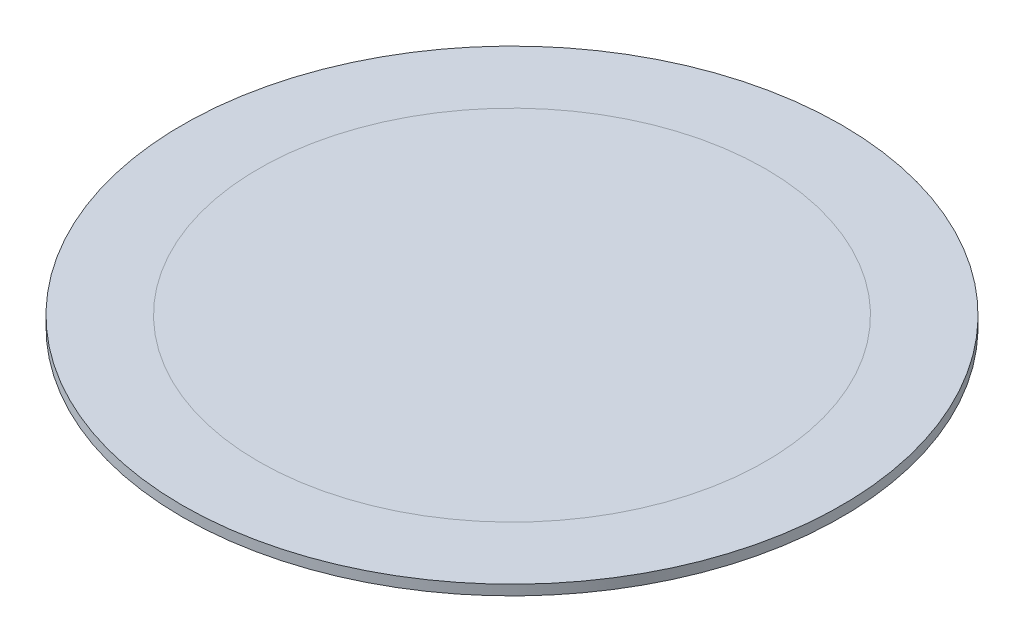
from build123d import *

# Parameters (mm, degrees)
SKETCH1_R           = 32.5
SKETCH1_R_2         = 25
BOSS_EXTRUDE1_DEPTH = 1
SKETCH2_R           = 25
BOSS_EXTRUDE2_DEPTH = 1


with BuildPart() as part:
    # Sketch1 → Boss-Extrude1 (new body)
    with BuildSketch(Plane(origin=(0, 0, 0), x_dir=(1, 0, 0), z_dir=(0, 1, 0))):
        with Locations(Location((0, 0, 0), (0, 0, 270))):
            Circle(SKETCH1_R)
        with Locations(Location((0, 0, 0), (0, 0, 270))):
            Circle(SKETCH1_R_2, mode=Mode.SUBTRACT)
    extrude(amount=BOSS_EXTRUDE1_DEPTH)


with BuildPart() as body_2:
    # Sketch2 → Boss-Extrude2 (new body)
    with BuildSketch(Plane.XZ):
        with Locations(Location((0, 0, 0), (0, 0, 270))):
            Circle(SKETCH2_R)
    extrude(amount=-BOSS_EXTRUDE2_DEPTH)


solid = Compound([part.part, body_2.part])
